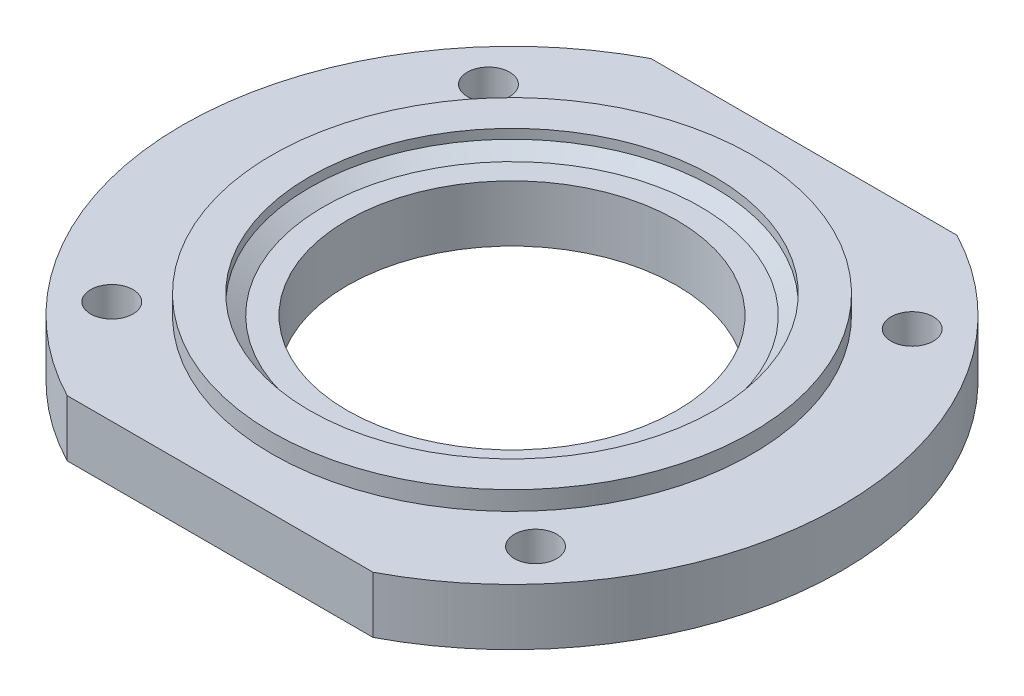
from build123d import *

# Parameters (mm, degrees)
F_4_5_4_5_DIAMETER_HOLE1_D     = 4.5
F_4_5_4_5_DIAMETER_HOLE1_DEPTH = 18
F_4_5_4_5_DIAMETER_HOLE1_TIP   = 1.351936393
SKETCH4_OUTSIDE_W              = 91.864
SKETCH4_OUTSIDE_H              = 91.864
SKETCH4_OUTSIDE_W_2            = 83.56481814
SKETCH4_OUTSIDE_H_2            = 62
CUT_EXTRUDE1_DEPTH             = 51.139804547


with BuildPart() as part:
    # Sketch1 → Revolve1 (revolve)
    with BuildSketch(Plane.XY, mode=Mode.PRIVATE) as revolve1_sk:
        Polygon((17.5, 0), (35, 0), (35, 6), (25.5, 6), (25.5, 8), (21.5, 8), (21.5, 7), (20, 6), (17.5, 6), align=None)
    revolve(revolve1_sk.sketch.rotate(Axis((0, 112.43124941, 0), (0, -1, 0)), 90), axis=Axis((0, 112.43124941, 0), (0, -1, 0)))

    # Ø4.5 (4.5) Diameter Hole1
    with Locations(Plane(origin=(0, 0, 0), x_dir=(-1, 0, 0), z_dir=(0, -1, 0))):
        with Locations((-22.5, 20), (-22.5, -20), (22.5, 20), (22.5, -20)):
            Hole(F_4_5_4_5_DIAMETER_HOLE1_D / 2, depth=F_4_5_4_5_DIAMETER_HOLE1_DEPTH)
            with Locations((0, 0, -(F_4_5_4_5_DIAMETER_HOLE1_DEPTH + F_4_5_4_5_DIAMETER_HOLE1_TIP / 2))):  # 118° drill point
                Cone(0, F_4_5_4_5_DIAMETER_HOLE1_D / 2, F_4_5_4_5_DIAMETER_HOLE1_TIP, mode=Mode.SUBTRACT)

    # Sketch4 outside → Cut-Extrude1 (cut, through all)
    with BuildSketch(Plane.XZ):
        Rectangle(SKETCH4_OUTSIDE_W, SKETCH4_OUTSIDE_H)
        Rectangle(SKETCH4_OUTSIDE_W_2, SKETCH4_OUTSIDE_H_2, mode=Mode.SUBTRACT)
    extrude(amount=-CUT_EXTRUDE1_DEPTH, mode=Mode.SUBTRACT)


solid = part.part
